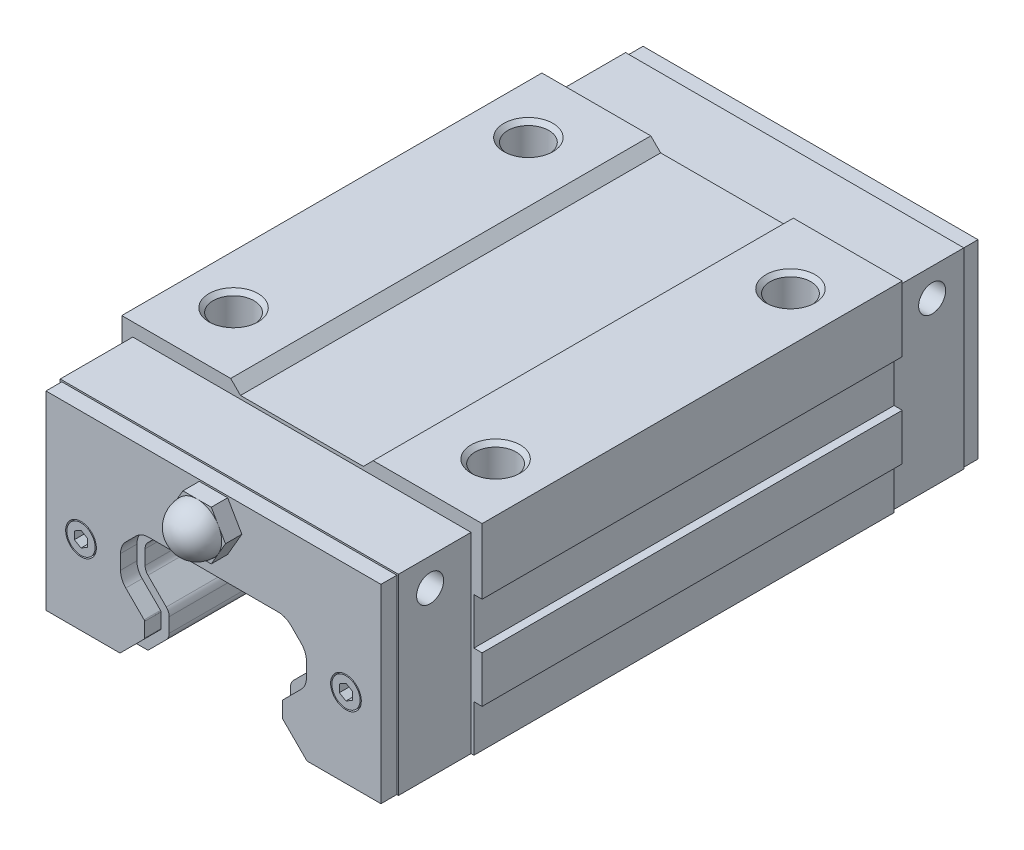
from build123d import *

# Parameters (mm, degrees)
BOSS_EXTRUDE1_START   = -36.45
SKETCH3_W             = 44
SKETCH3_H             = 23.4
BOSS_EXTRUDE1_DEPTH   = 72.9
SKETCH5_W             = 44
SKETCH5_H             = 51.3
EXTRUDE_1_DEPTH       = 25
CUT_EXTRUDE1_START    = -36.45
SKETCH4_W             = 1
SKETCH4_H             = 5.666666667
SKETCH4_H_2           = 17
CUT_EXTRUDE1_DEPTH    = 72.9
CUT_EXTRUDE_1_REACH   = 72.466
SKETCH24_W            = 1.35
SKETCH24_H            = 25
CUT_EXTRUDE6_DEPTH    = 10.8
CUT_EXTRUDE7_DEPTH    = 1.933333333
CUT_EXTRUDE2_START    = 36.45
CUT_EXTRUDE2_DEPTH    = 72.9
CUT_EXTRUDE3_DEPTH    = 2
THREADED_HOLE_1_D     = 5
THREADED_HOLE_1_DEPTH = 6
THREADED_HOLE_1_TIP   = 1.502151548
CHAMFER1_SIZE         = 0.5
SKETCH19_R            = 1.875
SKETCH19_R_2          = 1.725
CUT_EXTRUDE4_DEPTH    = 2
SKETCH20_R            = 1.65
CUT_EXTRUDE5_DEPTH    = 3
BOSS_EXTRUDE2_DEPTH   = 2


with BuildPart() as part:
    # Sketch3 → Boss-Extrude1 (new body)
    with BuildSketch(Plane.XY.offset(BOSS_EXTRUDE1_START)):
        with Locations((0, 11.7)):
            Rectangle(SKETCH3_W, SKETCH3_H)
    extrude(amount=BOSS_EXTRUDE1_DEPTH)

    # Sketch5 → 凸台-拉伸1 (add)
    with BuildSketch(Plane(origin=(0, 0, 0), x_dir=(1, 0, 0), z_dir=(0, 1, 0))):
        Rectangle(SKETCH5_W, SKETCH5_H)
    extrude(amount=EXTRUDE_1_DEPTH)

    # Sketch4 → Cut-Extrude1 (cut)
    with BuildSketch(Plane.XY.offset(CUT_EXTRUDE1_START)):
        with Locations((21.5, 2.833333334)):
            Rectangle(SKETCH4_W, SKETCH4_H)
        with Locations((21.5, 14.166666666)):
            Rectangle(SKETCH4_W, SKETCH4_H)
        with Locations((-21.5, 8.5)):
            Rectangle(SKETCH4_W, SKETCH4_H_2)
    extrude(amount=CUT_EXTRUDE1_DEPTH, mode=Mode.SUBTRACT)

    # Sketch6 → 切除-拉伸1 (cut, up to next)
    with BuildSketch(Plane.XY.offset(25.65), mode=Mode.PRIVATE) as cut_extrude_1_sk1:
        Polygon((-8.7, 25), (-7.5, 23.8), (7.5, 23.8), (8.7, 25), align=None)
    cut_extrude_1_tool1 = extrude(cut_extrude_1_sk1.sketch, amount=-CUT_EXTRUDE_1_REACH, mode=Mode.PRIVATE) & part.part
    add(cut_extrude_1_tool1.solids().sort_by_distance((0, 24.414815, 25.65))[0], mode=Mode.SUBTRACT)

    # Sketch24 → Cut-Extrude6 (cut)
    with BuildSketch(Plane.XY.offset(36.45)):
        with Locations((-21.325, 12.5)):
            Rectangle(SKETCH24_W, SKETCH24_H)
        with Locations((21.325, 12.5)):
            Rectangle(SKETCH24_W, SKETCH24_H)
    cut_extrude6 = extrude(amount=-CUT_EXTRUDE6_DEPTH, mode=Mode.SUBTRACT)

    # Sketch25 → Cut-Extrude7 (cut)
    with BuildSketch(Plane.XY.offset(36.45)):
        Polygon((-20.65, 0), (-20.65, 23.4), (20.65, 23.4), (20.65, 0), (20.45, 0), (20.45, 23.2), (-20.45, 23.2), (-20.45, 0), align=None)
    cut_extrude7 = extrude(amount=-CUT_EXTRUDE7_DEPTH, mode=Mode.SUBTRACT)

    # Sketch7 → Cut-Extrude2 (cut)
    with BuildSketch(Plane.XY.offset(CUT_EXTRUDE2_START)):
        with BuildLine():
            Line((-10, 0), (-7.7627417, 2.2372583))
            ThreePointArc((-7.7627417, 2.2372583), (-7.502614398, 2.626566319), (-7.411269837, 3.085786438))
            Line((-7.411269837, 3.085786438), (-7.411269837, 4.851471863))
            ThreePointArc((-7.411269837, 4.851471863), (-7.502614398, 5.310691981), (-7.7627417, 5.7))
            Line((-7.7627417, 5.7), (-10, 7.9372583))
            ThreePointArc((-10, 7.9372583), (-10.260127302, 8.326566319), (-10.351471863, 8.785786438))
            Line((-10.351471863, 8.785786438), (-10.351471863, 10.551471863))
            ThreePointArc((-10.351471863, 10.551471863), (-10.260127302, 11.010691981), (-10, 11.4))
            Line((-10, 11.4), (-8.751471863, 12.648528137))
            ThreePointArc((-8.751471863, 12.648528137), (-8.362163844, 12.908655439), (-7.902943725, 13))
            Line((-7.902943725, 13), (7.902943725, 13))
            ThreePointArc((7.902943725, 13), (8.362163844, 12.908655439), (8.751471863, 12.648528137))
            Line((8.751471863, 12.648528137), (10, 11.4))
            ThreePointArc((10, 11.4), (10.260127302, 11.010691981), (10.351471863, 10.551471863))
            Line((10.351471863, 10.551471863), (10.351471863, 8.785786438))
            ThreePointArc((10.351471863, 8.785786438), (10.260127302, 8.326566319), (10, 7.9372583))
            Line((10, 7.9372583), (7.7627417, 5.7))
            ThreePointArc((7.7627417, 5.7), (7.502614398, 5.310691981), (7.411269837, 4.851471863))
            Line((7.411269837, 4.851471863), (7.411269837, 3.085786438))
            ThreePointArc((7.411269837, 3.085786438), (7.502614398, 2.626566319), (7.7627417, 2.2372583))
            Line((7.7627417, 2.2372583), (10, 0))
            Line((10, 0), (-10, 0))
        make_face()
    extrude(amount=-CUT_EXTRUDE2_DEPTH, mode=Mode.SUBTRACT)

    # Sketch8 → Cut-Extrude3 (cut)
    with BuildSketch(Plane.XY.offset(36.45)):
        with BuildLine():
            Line((-7.7627417, 2.2372583), (-10, 0))
            Line((-10, 0), (-11.414213562, 0))
            Line((-11.414213562, 0), (-10.707106781, 0.707106781))
            Line((-10.707106781, 0.707106781), (-8.469848481, 2.944365081))
            ThreePointArc((-8.469848481, 2.944365081), (-8.426493931, 3.009249751), (-8.411269837, 3.085786438))
            Line((-8.411269837, 3.085786438), (-8.411269837, 4.851471863))
            ThreePointArc((-8.411269837, 4.851471863), (-8.426493931, 4.928008549), (-8.469848481, 4.992893219))
            Line((-8.469848481, 4.992893219), (-10.707106781, 7.230151519))
            ThreePointArc((-10.707106781, 7.230151519), (-11.184006834, 7.943882886), (-11.351471863, 8.785786438))
            Line((-11.351471863, 8.785786438), (-11.351471863, 10.551471863))
            ThreePointArc((-11.351471863, 10.551471863), (-11.184006834, 11.393375414), (-10.707106781, 12.107106781))
            Line((-10.707106781, 12.107106781), (-9.458578644, 13.355634919))
            ThreePointArc((-9.458578644, 13.355634919), (-8.744847276, 13.832534972), (-7.902943725, 14))
            Line((-7.902943725, 14), (7.902943725, 14))
            ThreePointArc((7.902943725, 14), (8.744847276, 13.832534972), (9.458578644, 13.355634919))
            Line((9.458578644, 13.355634919), (10.707106781, 12.107106781))
            ThreePointArc((10.707106781, 12.107106781), (11.184006834, 11.393375414), (11.351471863, 10.551471863))
            Line((11.351471863, 10.551471863), (11.351471863, 8.785786438))
            ThreePointArc((11.351471863, 8.785786438), (11.184006834, 7.943882886), (10.707106781, 7.230151519))
            Line((10.707106781, 7.230151519), (8.469848481, 4.992893219))
            ThreePointArc((8.469848481, 4.992893219), (8.426493931, 4.928008549), (8.411269837, 4.851471863))
            Line((8.411269837, 4.851471863), (8.411269837, 3.085786438))
            ThreePointArc((8.411269837, 3.085786438), (8.426493931, 3.009249751), (8.469848481, 2.944365081))
            Line((8.469848481, 2.944365081), (10.707106781, 0.707106781))
            Line((10.707106781, 0.707106781), (11.414213562, 0))
            Line((11.414213562, 0), (10, 0))
            Line((10, 0), (7.7627417, 2.2372583))
            ThreePointArc((7.7627417, 2.2372583), (7.502614398, 2.626566319), (7.411269837, 3.085786438))
            Line((7.411269837, 3.085786438), (7.411269837, 4.851471863))
            ThreePointArc((7.411269837, 4.851471863), (7.502614398, 5.310691981), (7.7627417, 5.7))
            Line((7.7627417, 5.7), (10, 7.9372583))
            ThreePointArc((10, 7.9372583), (10.260127302, 8.326566319), (10.351471863, 8.785786438))
            Line((10.351471863, 8.785786438), (10.351471863, 10.551471863))
            ThreePointArc((10.351471863, 10.551471863), (10.260127302, 11.010691981), (10, 11.4))
            Line((10, 11.4), (8.751471863, 12.648528137))
            ThreePointArc((8.751471863, 12.648528137), (8.362163844, 12.908655439), (7.902943725, 13))
            Line((7.902943725, 13), (-7.902943725, 13))
            ThreePointArc((-7.902943725, 13), (-8.362163844, 12.908655439), (-8.751471863, 12.648528137))
            Line((-8.751471863, 12.648528137), (-10, 11.4))
            ThreePointArc((-10, 11.4), (-10.260127302, 11.010691981), (-10.351471863, 10.551471863))
            Line((-10.351471863, 10.551471863), (-10.351471863, 8.785786438))
            ThreePointArc((-10.351471863, 8.785786438), (-10.260127302, 8.326566319), (-10, 7.9372583))
            Line((-10, 7.9372583), (-7.7627417, 5.7))
            ThreePointArc((-7.7627417, 5.7), (-7.502614398, 5.310691981), (-7.411269837, 4.851471863))
            Line((-7.411269837, 4.851471863), (-7.411269837, 3.085786438))
            ThreePointArc((-7.411269837, 3.085786438), (-7.502614398, 2.626566319), (-7.7627417, 2.2372583))
        make_face()
    cut_extrude3 = extrude(amount=-CUT_EXTRUDE3_DEPTH, mode=Mode.SUBTRACT)

    # Mirror1: Cut-Extrude6, Cut-Extrude7, Cut-Extrude3 across plane
    add(cut_extrude6.mirror(Plane.XY), mode=Mode.SUBTRACT)
    add(cut_extrude7.mirror(Plane.XY), mode=Mode.SUBTRACT)
    add(cut_extrude3.mirror(Plane.XY), mode=Mode.SUBTRACT)

    # threaded hole 1
    with Locations(Plane(origin=(0, 25, 0), x_dir=(-1, 0, 0), z_dir=(0, 1, 0))):
        with Locations((16, 18), (-16, -18), (16, -18), (-16, 18)):
            Hole(THREADED_HOLE_1_D / 2, depth=THREADED_HOLE_1_DEPTH)
            with Locations((0, 0, -(THREADED_HOLE_1_DEPTH + THREADED_HOLE_1_TIP / 2))):  # 118° drill point
                Cone(0, THREADED_HOLE_1_D / 2, THREADED_HOLE_1_TIP, mode=Mode.SUBTRACT)

    # Chamfer1
    chamfer1_edges = [part.edges().sort_by_distance(p)[0] for p in [
        (13.5, 25, 18),
        (-18.5, 25, -18),
        (13.5, 25, -18),
        (-18.5, 25, 18),
    ]]
    chamfer(chamfer1_edges, length=CHAMFER1_SIZE)

    # Sketch19 → Cut-Extrude4 (cut)
    # profile 1 of 4: a face of its own
    with BuildSketch(Plane.XY.offset(36.45)):
        with Locations((-16.175735931, 9.66862915)):
            Circle(SKETCH19_R)
        with Locations((-16.175735931, 9.66862915)):
            Circle(SKETCH19_R_2, mode=Mode.SUBTRACT)
    # profile 2 of 4: a face of its own
    with BuildSketch(Plane.XY.offset(36.45)):
        Polygon((-15.363837115, 9.19987915), (-15.363837115, 10.13737915), (-16.175735931, 10.60612915), (-16.987634747, 10.13737915), (-16.987634747, 9.19987915), (-16.175735931, 8.73112915), align=None)
    # profile 3 of 4: a face of its own
    with BuildSketch(Plane.XY.offset(36.45)):
        with Locations((16.175735931, 9.66862915)):
            Circle(SKETCH19_R)
        with Locations((16.175735931, 9.66862915)):
            Circle(SKETCH19_R_2, mode=Mode.SUBTRACT)
    # profile 4 of 4: a face of its own
    with BuildSketch(Plane.XY.offset(36.45)):
        Polygon((16.175735931, 10.60612915), (16.987634747, 10.13737915), (16.987634747, 9.19987915), (16.175735931, 8.73112915), (15.363837115, 9.19987915), (15.363837115, 10.13737915), align=None)
    cut_extrude4 = extrude(amount=-CUT_EXTRUDE4_DEPTH, mode=Mode.SUBTRACT)

    # Mirror2: Cut-Extrude4 across plane
    add(cut_extrude4.mirror(Plane.XY), mode=Mode.SUBTRACT)

    # Sketch20 → Cut-Extrude5 (cut)
    with BuildSketch(Plane(origin=(21, 0, 0), x_dir=(0, 0, -1), z_dir=(1, 0, 0))):
        with Locations((-30.65, 20)):
            Circle(SKETCH20_R)
        with Locations((30.65, 20)):
            Circle(SKETCH20_R)
    cut_extrude5 = extrude(amount=-CUT_EXTRUDE5_DEPTH, mode=Mode.SUBTRACT)

    # Sketch22 → Boss-Extrude2 (add)
    with BuildSketch(Plane.XY.offset(36.45)):
        Polygon((1.732050808, 23), (-1.732050808, 23), (-3.464101615, 20), (-1.732050808, 17), (1.732050808, 17), (3.464101615, 20), align=None)
    extrude(amount=BOSS_EXTRUDE2_DEPTH)

    # Sketch23 → Revolve1 (revolve)
    with BuildSketch(Plane(origin=(0, 0, 0), x_dir=(0, 0, -1), z_dir=(1, 0, 0))):
        with BuildLine():
            Line((-38.45, 20), (-38.45, 23))
            ThreePointArc((-38.45, 23), (-40.571320344, 22.121320344), (-41.45, 20))
            Line((-41.45, 20), (-38.45, 20))
        make_face()
    revolve(axis=Axis((0, 20, 38.45), (0, 0, 1)))

    # Mirror3: Cut-Extrude5 across plane
    add(cut_extrude5.mirror(Plane(origin=(0, 0, 0), x_dir=(0, 0, 1), z_dir=(1, 0, 0))), mode=Mode.SUBTRACT)


solid = part.part
